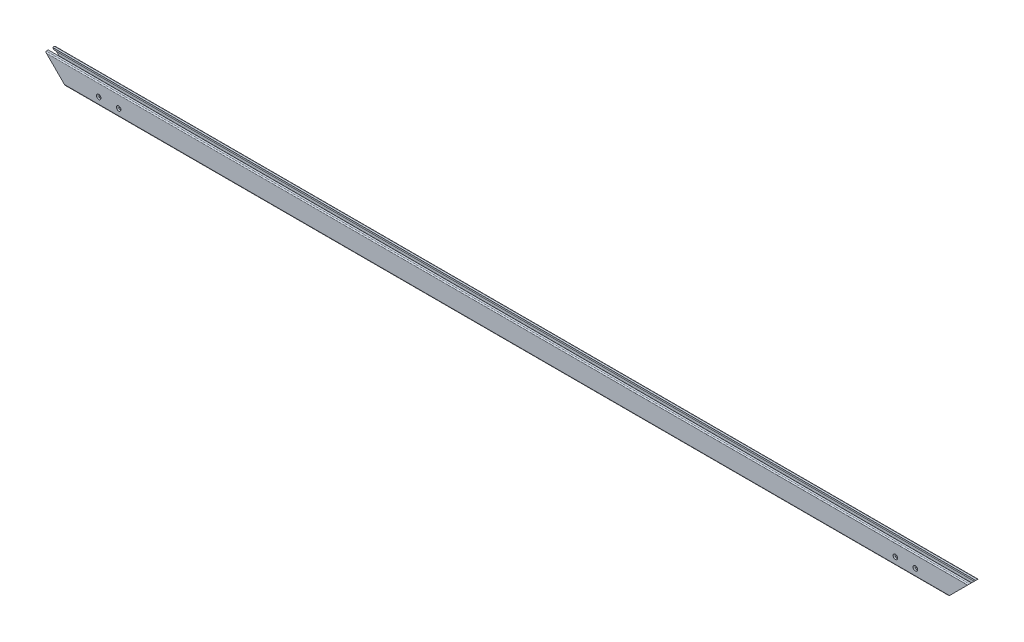
SolidWorks part; units mm, degrees
ref_plane "前视" through (0, 0, 0) normal (0, 0, 1) x (1, 0, 0)
ref_plane "上视" through (0, 0, 0) normal (0, 1, 0) x (1, 0, 0)
ref_plane "右视" through (0, 0, 0) normal (1, 0, 0) x (0, 0, -1)
sketch3d "3D草图1"
  line L0 (-693, 0, 0) -> (693, 0, 0)
  dimension "D1" = 1386
other "结构构件1"
ref_plane "基准面1" through (-693, 0, 0) normal (1, 0, 0) x (0, 0, -1)
sketch "Sketch11" plane through (-693, 0, 0) normal (1, 0, 0) x (0, 0, -1)
  line L1 (0, 16.311) -> (0, -16.311) construction
  line L2 (0, 0) -> (9.513, 0) construction
  line L3 (-6, -15) -> (-3.25, -15)
  line L4 (-7.5, -13.5) -> (-7.5, 13.5)
  line L5 (-6, 15) -> (-3.25, 15)
  line L6 (7.5, -13.5) -> (7.5, 13.5)
  line L17 (3.25, 15) -> (6, 15)
  line L20 (-5, 12.7) -> (-5, 7)
  line L21 (-3.25, 12.7) -> (-5, 12.7)
  line L24 (5, 12.7) -> (5, 7)
  line L25 (3.25, 12.7) -> (5, 12.7)
  line L26 (-3.25, 15) -> (-3.25, 12.7)
  line L27 (3.25, 15) -> (3.25, 12.7)
  line L40 (5, -12.7) -> (5, -7)
  line L41 (3.25, -12.7) -> (5, -12.7)
  line L44 (-5, -12.7) -> (-5, -7)
  line L45 (-3.25, -12.7) -> (-5, -12.7)
  line L47 (3.25, -15) -> (3.25, -12.7)
  line L48 (-3.25, -15) -> (-3.25, -12.7)
  line L49 (3.25, -15) -> (6, -15)
  arc A0 (-6, -15) -> (-7.5, -13.5) centre (-6, -13.5) cw
  arc A1 (6, -15) -> (7.5, -13.5) centre (6, -13.5) ccw
  arc A2 (6, 15) -> (7.5, 13.5) centre (6, 13.5) cw
  arc A3 (-7.5, 13.5) -> (-6, 15) centre (-6, 13.5) cw
  circle A4 centre (0, 0) radius 2.5
  arc A5 (-5, 7) -> (5, 7) centre (0, 10.3166) ccw
  arc A6 (-5, -7) -> (5, -7) centre (0, -10.3166) cw
  point P4 (0, 0)
  point P21 (0, 0)
  point P44 (-7.5, 15)
  point P45 (7.5, 15)
  point P46 (7.5, -15)
  point P47 (-7.5, -15)
  point P48 (0, -15)
  point P49 (0, 15)
  dimension "D1" = 30
  dimension "D2" = 15
  dimension "D3" = 1.5
  dimension "D4" = 5
  dimension "D5" = 6.5
  dimension "D6" = 6
  dimension "D7" = 8
  dimension "D8" = 10
  dimension "D9" = 2.3
sketch "草图4" plane through (0, 0, 7.5) normal (0, 0, 1) x (1, 0, 0)
  line L0 (-693, 15) -> (-663, -15)
  line L1 (693, -15) -> (-693, -15) construction
  line L2 (0, 0) -> (0, -85.0329) construction
  line L3 (-663, -15) -> (-693, -15)
  line L4 (-693, -15) -> (-693, 15)
  line L5 (693, -15) -> (693, 15)
  line L6 (663, -15) -> (693, -15)
  line L7 (693, 15) -> (663, -15)
extrude "切除-拉伸1" cut sketch "草图4" against normal through all
hole_wizard "M8 螺纹孔1" positions "草图6" profile "草图7" tap size "M8" standard "Iso" end condition through all
sketch "草图6" plane through (0, 0, 7.5) normal (0, 0, 1) x (1, 0, 0)
  line L0 (0, 0) -> (0, -60.6345) construction
  line L2 (693, 15) -> (-693, 15) construction
  point P0 (-613, -4)
  point P2 (-583, -4)
  point P9 (583, -4)
  point P10 (613, -4)
  dimension "D1" = 30
  dimension "D2" = 19
  dimension "D3" = 80
sketch "草图7" plane through (-613, -4, 7.5) normal (1, 0, 0) x (0, -1, 0)
  line L0 (0, 0) -> (0, 15)
  line L1 (0, 15) -> (3.4, 15)
  line L2 (3.4, 15) -> (3.4, 0)
  line L5 (3.4, 0) -> (0, 0)
  line L11 (0, -6.35) -> (0, 107.95) construction
  dimension "通孔螺纹孔钻头直径" = 6.8
  dimension "通孔螺纹孔钻头深度" = 15
cosmetic thread "孔螺蚊线1" parameters "D2"=8
cosmetic thread "孔螺蚊线2" parameters "D2"=8
cosmetic thread "孔螺蚊线3" parameters "D2"=8
cosmetic thread "孔螺蚊线4" parameters "D2"=8
